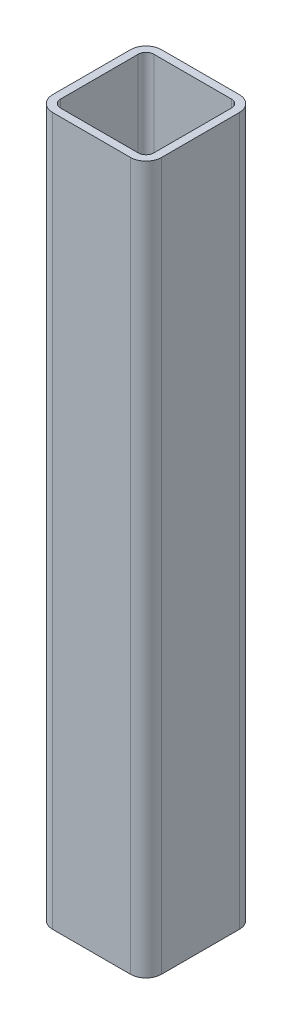
from build123d import *

# Parameters (mm, degrees)
GB_T6728_2002_70_70_5_1_DEPTH = 455


with BuildPart() as part:
    # Sketch1 → 结构用冷弯空心方钢(gb t6728-2002) 70×70×5(1) (new body)
    with BuildSketch(Plane(origin=(0, 0, 0), x_dir=(-1, 0, 0), z_dir=(0, 1, 0))):
        with BuildLine():
            Line((-25, -35), (25, -35))
            ThreePointArc((25, -35), (32.071067812, -32.071067812), (35, -25))
            Line((35, -25), (35, 25))
            ThreePointArc((35, 25), (32.071067812, 32.071067812), (25, 35))
            Line((25, 35), (-25, 35))
            ThreePointArc((-25, 35), (-32.071067812, 32.071067812), (-35, 25))
            Line((-35, 25), (-35, -25))
            ThreePointArc((-35, -25), (-32.071067812, -32.071067812), (-25, -35))
        make_face()
        with BuildLine():
            Line((-25, -30), (25, -30))
            ThreePointArc((25, -30), (28.535533906, -28.535533906), (30, -25))
            Line((30, -25), (30, 25))
            ThreePointArc((30, 25), (28.535533906, 28.535533906), (25, 30))
            Line((25, 30), (-25, 30))
            ThreePointArc((-25, 30), (-28.535533906, 28.535533906), (-30, 25))
            Line((-30, 25), (-30, -25))
            ThreePointArc((-30, -25), (-28.535533906, -28.535533906), (-25, -30))
        make_face(mode=Mode.SUBTRACT)
    extrude(amount=GB_T6728_2002_70_70_5_1_DEPTH)


solid = part.part
